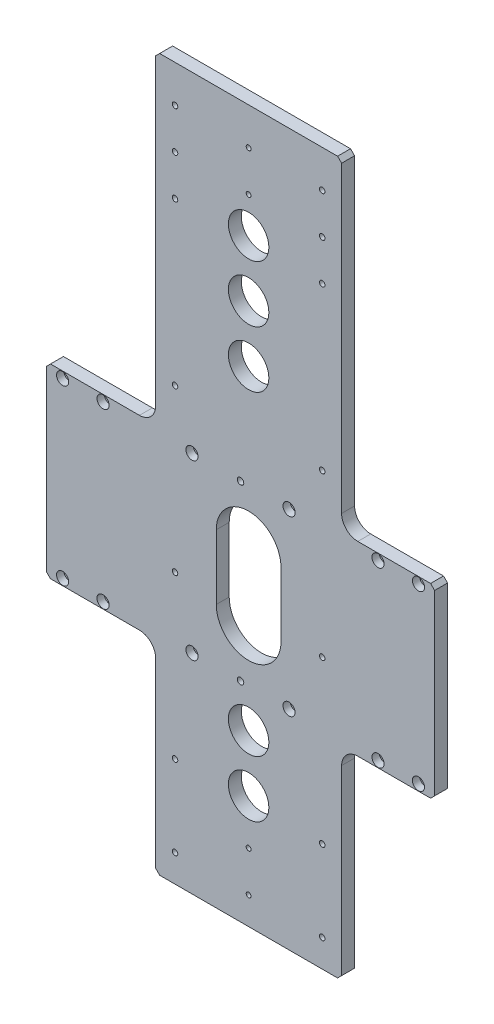
SolidWorks part; units mm, degrees
material "6061 合金"
ref_plane "Front" through (0, 0, 0) normal (0, 0, 1) x (1, 0, 0)
ref_plane "Top" through (0, 0, 0) normal (0, 1, 0) x (1, 0, 0)
ref_plane "Right" through (0, 0, 0) normal (1, 0, 0) x (0, 0, -1)
sketch "草图1" plane through (0, 0, 0) normal (0, 0, 1) x (1, 0, 0)
  line L1 (-240, -115) -> (240, -115)
  line L2 (-240, -115) -> (-240, 115)
  line L3 (-240, 115) -> (240, 115)
  line L4 (240, -115) -> (240, 115)
  line L5 (-240, -115) -> (240, 115) construction
  line L6 (-240, 115) -> (240, -115) construction
  line L7 (-105, 515) -> (125, 515)
  line L8 (-105, 515) -> (-105, 115)
  line L9 (-105, 115) -> (125, 115)
  line L10 (125, 515) -> (125, 115)
  line L11 (-105, 515) -> (125, 115) construction
  line L12 (-105, 115) -> (125, 515) construction
  line L13 (-105, -365) -> (125, -365)
  line L14 (-105, -365) -> (-105, -115)
  line L15 (-105, -115) -> (125, -115)
  line L16 (125, -365) -> (125, -115)
  line L17 (-105, -365) -> (125, -115) construction
  line L18 (-105, -115) -> (125, -365) construction
  point P0 (0, 0)
  dimension "D1" = 230
  dimension "D2" = 480
  dimension "D3" = 230
  dimension "D4" = 400
  dimension "D5" = 250
  dimension "D6" = 115
extrude "凸台-拉伸1" add sketch "草图1" along normal blind 16 contours L10 L7 L8 L3 | L1 L4 L3 L2 | L13 L16 L1 L14
fillet "圆角1" radius 20 4 edges at (125, 115, 8) (125, -115, 8) (-105, -115, 8) (-105, 115, 8)
hole_wizard "打孔尺寸(%根据)内六角圆柱头螺钉的类型1" positions "草图2" profile "草图3" counterbore size "M8" standard "GB" end condition through all
sketch "草图2" plane through (0, 0, 16) normal (0, 0, 1) x (1, 0, 0)
  line L10 (-240, 0) -> (240, 0) construction
  line L11 (-240, -115) -> (-240, 115) construction
  line L12 (240, -115) -> (240, 115) construction
  line L14 (-220, -107) -> (220, -107) construction
  line L15 (-220, -107) -> (-220, 107) construction
  line L16 (-220, 107) -> (220, 107) construction
  line L17 (220, -107) -> (220, 107) construction
  line L18 (0, 107) -> (0, -107) construction
  line L19 (-220, 0) -> (220, 0) construction
  line L20 (-170, 107) -> (-170, -107) construction
  line L21 (170, 107) -> (170, -107) construction
  line L22 (-60, 107) -> (-60, -107) construction
  line L23 (60, 107) -> (60, -107) construction
  point P318 (220, 107)
  point P505 (-220, -107)
  point P506 (-220, 107)
  point P507 (220, -107)
  point P529 (-170, 107)
  point P530 (-170, -107)
  point P531 (170, 107)
  point P532 (170, -107)
  point P533 (-60, 107)
  point P534 (-60, -107)
  point P535 (60, 107)
  point P536 (60, -107)
  dimension "D1" = 214
  dimension "D2" = 440
  dimension "D3" = 340
  dimension "D4" = 120
  dimension "D5" = 0
sketch "草图3" plane through (60, -107, 16) normal (1, 0, 0) x (0, -1, 0)
  line L0 (0, 0) -> (0, 16)
  line L1 (0, 16) -> (4.5, 16)
  line L3 (4.5, 16) -> (4.5, 9)
  line L4 (4.5, 9) -> (7.5, 9)
  line L5 (7.5, 9) -> (7.5, 0)
  line L7 (7.5, 0) -> (0, 0)
  line L11 (0, -6.35) -> (0, 107.95) construction
  dimension "通孔孔直径" = 9
  dimension "通孔孔深度" = 16
  dimension "柱形沉头孔直径" = 15
  dimension "柱形沉头孔深度" = 9
hole_wizard "大小mm 暗销孔1" positions "草图4" profile "草图5" hole size "Ø8.0" standard "GB" end condition through all
sketch "草图4" plane through (0, 0, 16) normal (0, 0, 1) x (1, 0, 0)
  line L1 (-220, -107) -> (220, -107) construction
  line L2 (-220, -107) -> (-220, 107) construction
  line L3 (-220, 107) -> (220, 107) construction
  line L4 (220, -107) -> (220, 107) construction
  line L5 (0, 107) -> (0, -107) construction
  line L6 (-220, 0) -> (220, 0) construction
  line L7 (-240, 0) -> (240, 0) construction
  line L8 (-240, -115) -> (-240, 115) construction
  line L9 (240, -115) -> (240, 115) construction
  circle A0 centre (220, 107) radius 4.5 construction
  circle A1 centre (-220, 107) radius 4.5 construction
  point P769 (0, -107)
  point P771 (0, 107)
sketch "草图5" plane through (0, 107, 16) normal (1, 0, 0) x (0, -1, 0)
  line L0 (0, 0) -> (0, 16)
  line L1 (0, 16) -> (4, 16)
  line L2 (4, 16) -> (4, 0)
  line L5 (4, 0) -> (0, 0)
  line L11 (0, -6.35) -> (0, 107.95) construction
  dimension "通孔孔直径" = 8
  dimension "通孔孔深度" = 16
hole_wizard "M8 螺纹孔1" positions "草图6" profile "草图7" tap size "M8" standard "GB"
sketch "草图6" plane through (0, 0, 16) normal (0, 0, 1) x (1, 0, 0)
  line L1 (-81, -469) -> (101, -469) construction
  line L2 (-81, -469) -> (-81, 469) construction
  line L3 (-81, 469) -> (101, 469) construction
  line L4 (101, -469) -> (101, 469) construction
  line L5 (10, 469) -> (10, -469) construction
  line L6 (-81, 0) -> (101, 0) construction
  line L7 (10, 515) -> (10, -365) construction
  line L8 (-105, 515) -> (125, 515) construction
  line L9 (-105, -365) -> (125, -365) construction
  line L10 (-240, 0) -> (240, 0) construction
  line L11 (-240, -115) -> (-240, 115) construction
  line L12 (240, -115) -> (240, 115) construction
  line L13 (101, -469) -> (101, 469) construction
  point P2 (101, 469)
  point P562 (-81, 469)
  point P586 (-81, 169)
  point P588 (-81, 369)
  point P590 (-81, 419)
  point P595 (-81, -31)
  point P597 (-81, -231)
  point P599 (-81, -331)
  point P606 (101, -331)
  point P607 (101, -231)
  point P608 (101, -31)
  point P609 (101, 419)
  point P610 (101, 369)
  point P611 (101, 169)
  dimension "D1" = 182
  dimension "D2" = 200
  dimension "D3" = 46
  dimension "D4" = 50
  dimension "D5" = 50
  dimension "D6" = 200
  dimension "D7" = 200
  dimension "D8" = 100
sketch "草图7" plane through (101, 469, 16) normal (1, 0, 0) x (0, -1, 0)
  line L0 (0, 0) -> (0, 24.2929)
  line L1 (0, 24.2929) -> (3.4, 22.25)
  line L2 (3.4, 22.25) -> (3.4, 0)
  line L5 (3.4, 0) -> (0, 0)
  line L10 (0, 24.2929) -> (-3.4, 22.25) construction
  line L11 (0, -6.35) -> (0, 107.95) construction
  dimension "螺纹孔钻头直径" = 6.8
  dimension "螺纹孔钻头深度" = 22.25
  dimension "导头角度" = 118
cosmetic thread "孔螺蚊线2" parameters "D1"=16, "D2"=8
cosmetic thread "孔螺蚊线3" parameters "D1"=16, "D2"=8
cosmetic thread "孔螺蚊线4" parameters "D1"=16, "D2"=8
cosmetic thread "孔螺蚊线5" parameters "D1"=16, "D2"=8
cosmetic thread "孔螺蚊线6" parameters "D1"=16, "D2"=8
cosmetic thread "孔螺蚊线7" parameters "D1"=16, "D2"=8
cosmetic thread "孔螺蚊线8" parameters "D1"=16, "D2"=8
cosmetic thread "孔螺蚊线9" parameters "D1"=16, "D2"=8
cosmetic thread "孔螺蚊线10" parameters "D1"=16, "D2"=8
cosmetic thread "孔螺蚊线11" parameters "D1"=16, "D2"=8
cosmetic thread "孔螺蚊线12" parameters "D1"=16, "D2"=8
cosmetic thread "孔螺蚊线14" parameters "D1"=16, "D2"=8
cosmetic thread "孔螺蚊线15" parameters "D1"=16, "D2"=8
cosmetic thread "孔螺蚊线16" parameters "D1"=16, "D2"=8
chamfer "倒角2" distance 5 angle 45 4 edges at (125, -365, 8) (-105, -365, 8) (-105, 515, 8) (125, 515, 8)
chamfer "倒角3" distance 5 angle 45 4 edges at (240, 115, 8) (240, -115, 8) (-240, -115, 8) (-240, 115, 8)
sketch "草图8" plane through (0, 0, 16) normal (0, 0, 1) x (1, 0, 0)
  line L0 (10, 40) -> (10, -40) construction
  line L3 (10, 515) -> (10, -365) construction
  line L4 (-100, 515) -> (120, 515) construction
  line L5 (-100, -365) -> (120, -365) construction
  line L6 (50, 40) -> (50, -40)
  line L7 (-30, 40) -> (-30, -40)
  circle A2 centre (10, 375) radius 25
  circle A3 centre (10, 305) radius 25
  circle A5 centre (10, -155) radius 25
  circle A6 centre (10, -225) radius 25
  circle A7 centre (10, 235) radius 25
  arc A8 (50, 40) -> (-30, 40) centre (10, 40) ccw
  arc A9 (-30, -40) -> (50, -40) centre (10, -40) ccw
  point P2 (10, 0)
  dimension "D3" = 50
  dimension "D5" = 70
  dimension "D6" = 70
  dimension "D7" = 70
  dimension "D1" = 80
  dimension "D2" = 80
  dimension "D4" = 140
  dimension "D8" = 140
extrude "切除-拉伸1" cut sketch "草图8" against normal through all
hole_wizard "大小mm 暗销孔2" positions "草图9" profile "草图10" hole size "Ø6.0" standard "GB" end condition through all
sketch "草图9" plane through (0, 0, 16) normal (0, 0, 1) x (1, 0, 0)
  line L0 (101, 469) -> (-81, 469) construction
  line L1 (10, 469) -> (10, 419) construction
  line L2 (101, 419) -> (-81, 419) construction
  line L3 (101, -331) -> (-81, -331) construction
  line L4 (10, -331) -> (10, -281) construction
  line L5 (101, -231) -> (-81, -231) construction
  point P7 (10, 469)
  point P17 (10, 419)
  point P23 (10, -331)
  point P24 (10, -281)
  dimension "D1" = 50
sketch "草图10" plane through (10, -281, 16) normal (1, 0, 0) x (0, -1, 0)
  line L0 (0, 0) -> (0, 16)
  line L1 (0, 16) -> (3, 16)
  line L2 (3, 16) -> (3, 0)
  line L5 (3, 0) -> (0, 0)
  line L11 (0, -6.35) -> (0, 107.95) construction
  dimension "通孔孔直径" = 6
  dimension "通孔孔深度" = 16
